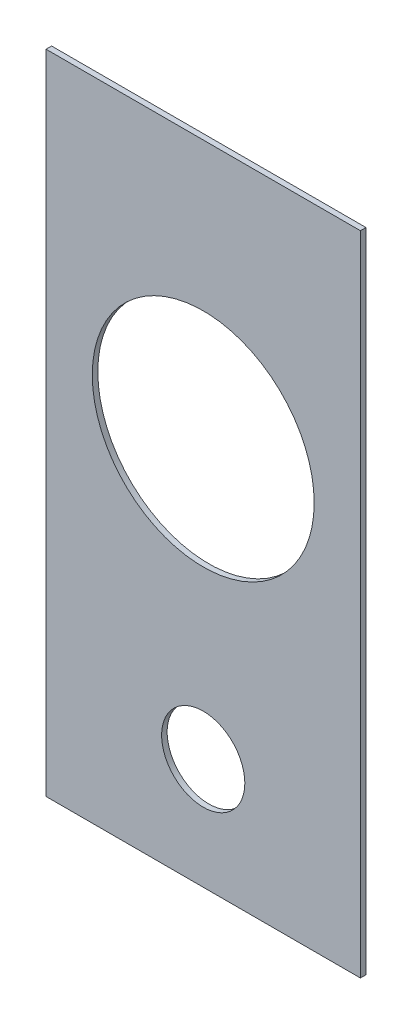
from build123d import *

# Parameters (mm, degrees)
SKETCH1_W           = 170
SKETCH1_H           = 350
SKETCH1_R           = 60
SKETCH1_R_2         = 22.5
BOSS_EXTRUDE1_DEPTH = 3


with BuildPart() as part:
    # Sketch1 → Boss-Extrude1 (new body)
    with BuildSketch(Plane.XY):
        with Locations((85, 175)):
            Rectangle(SKETCH1_W, SKETCH1_H)
        with Locations((85, 210)):
            Circle(SKETCH1_R, mode=Mode.SUBTRACT)
        with Locations((85, 60)):
            Circle(SKETCH1_R_2, mode=Mode.SUBTRACT)
    extrude(amount=BOSS_EXTRUDE1_DEPTH)


solid = part.part
